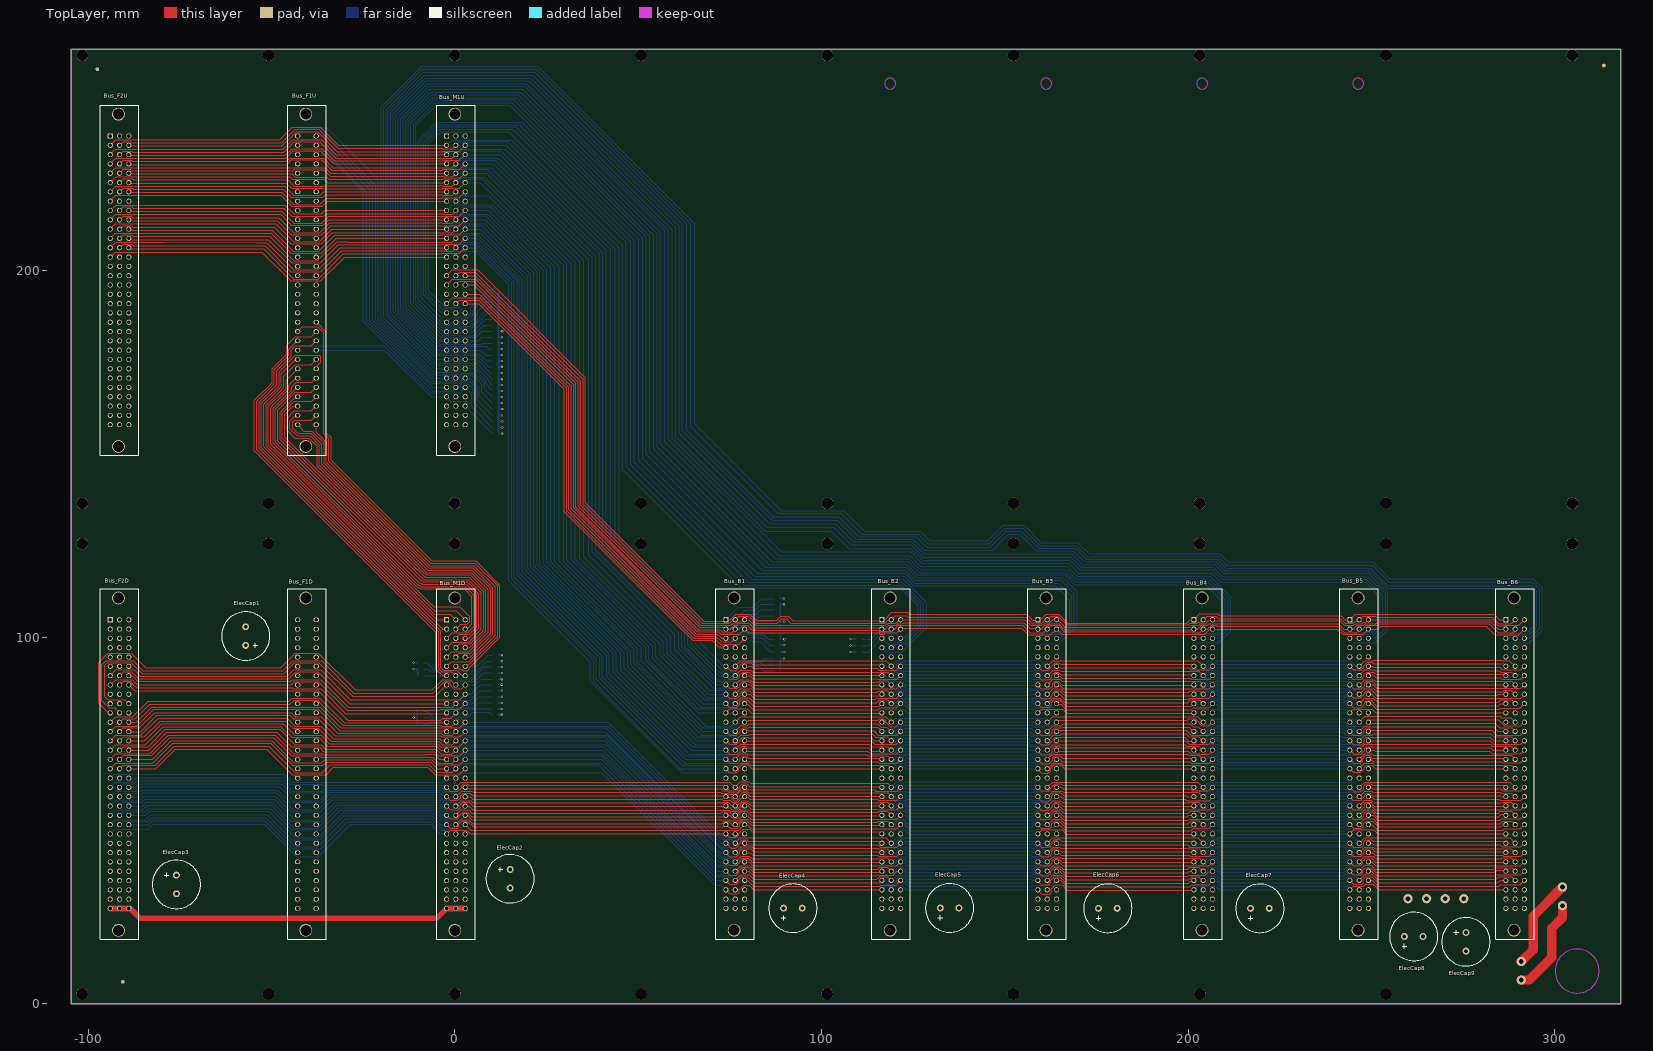
[diagram p0: TopLayer view]
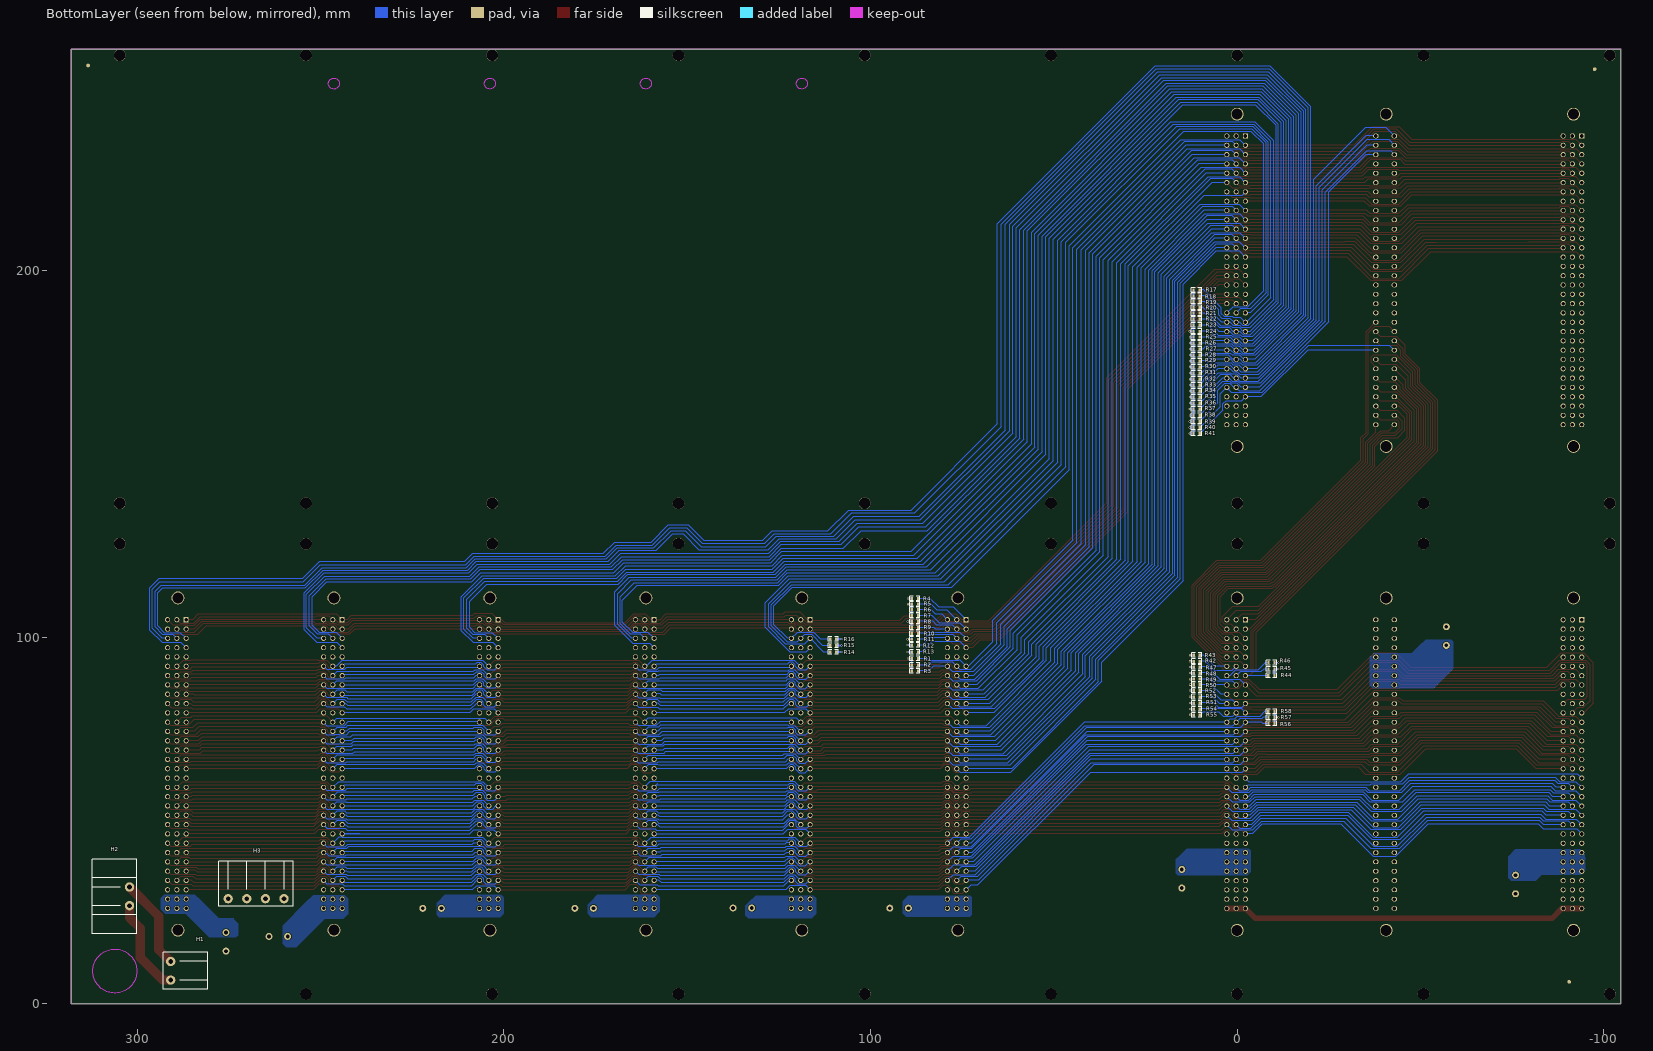
[diagram p1: BottomLayer view, seen from below]
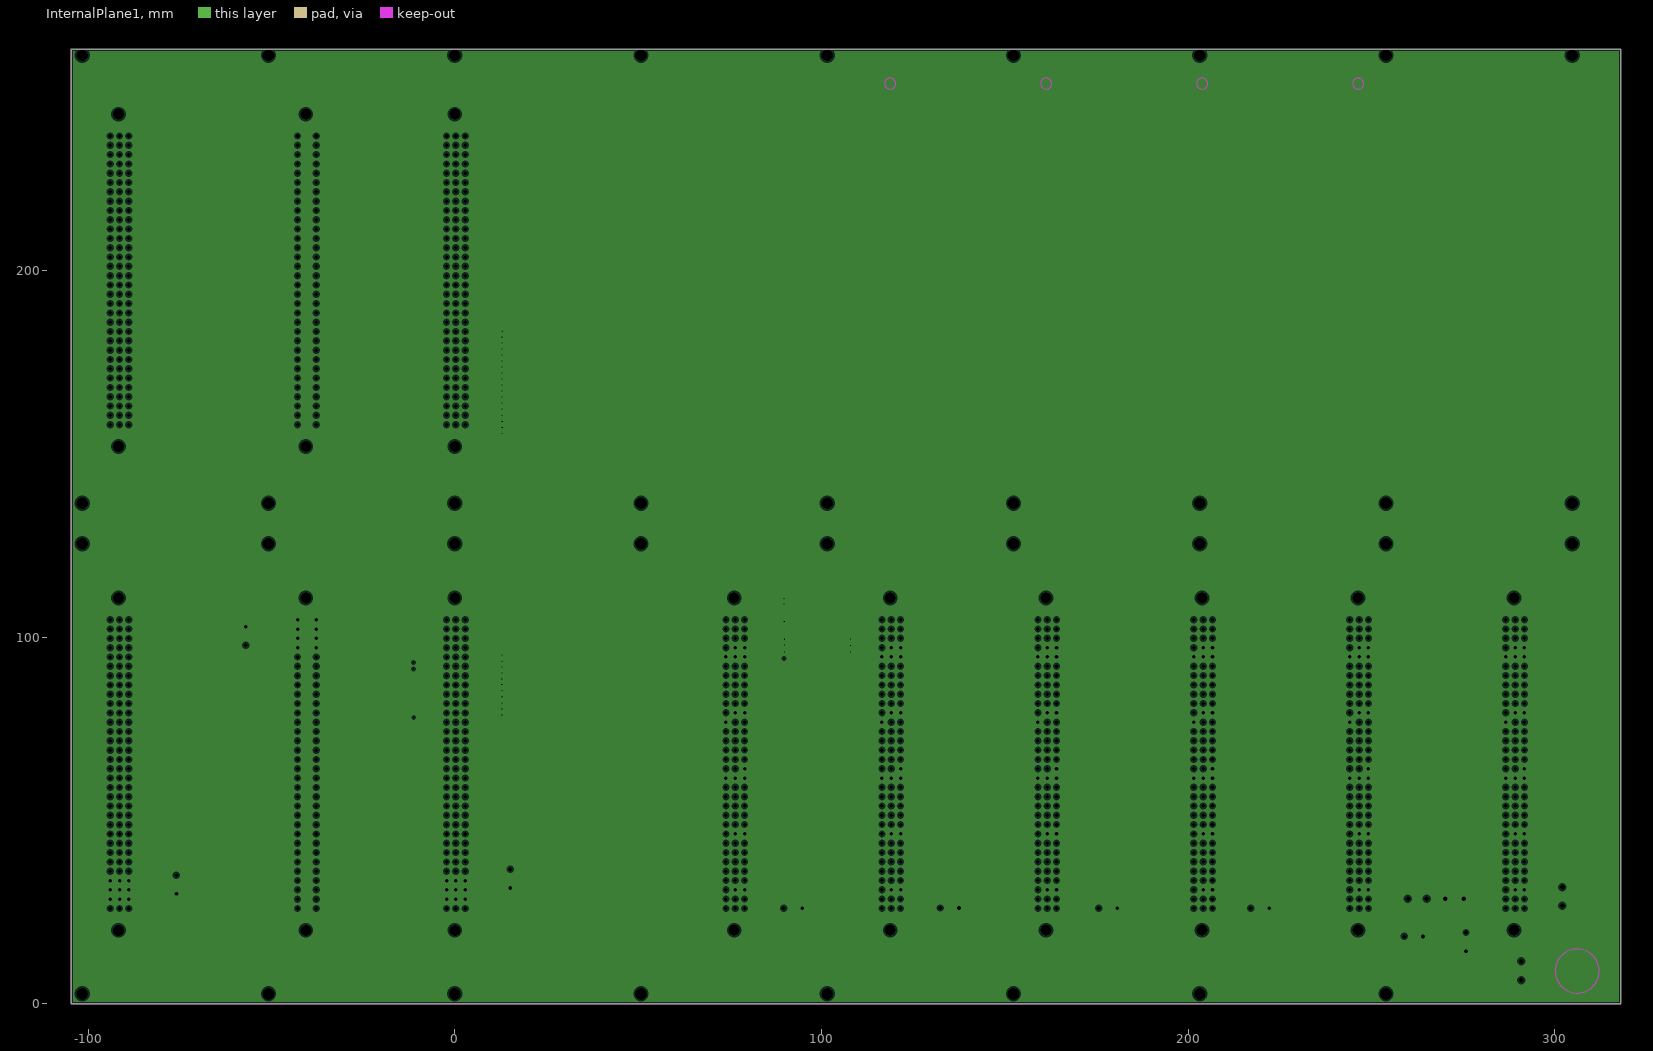
[diagram p2: InternalPlane1, clearances drawn from the general rule]
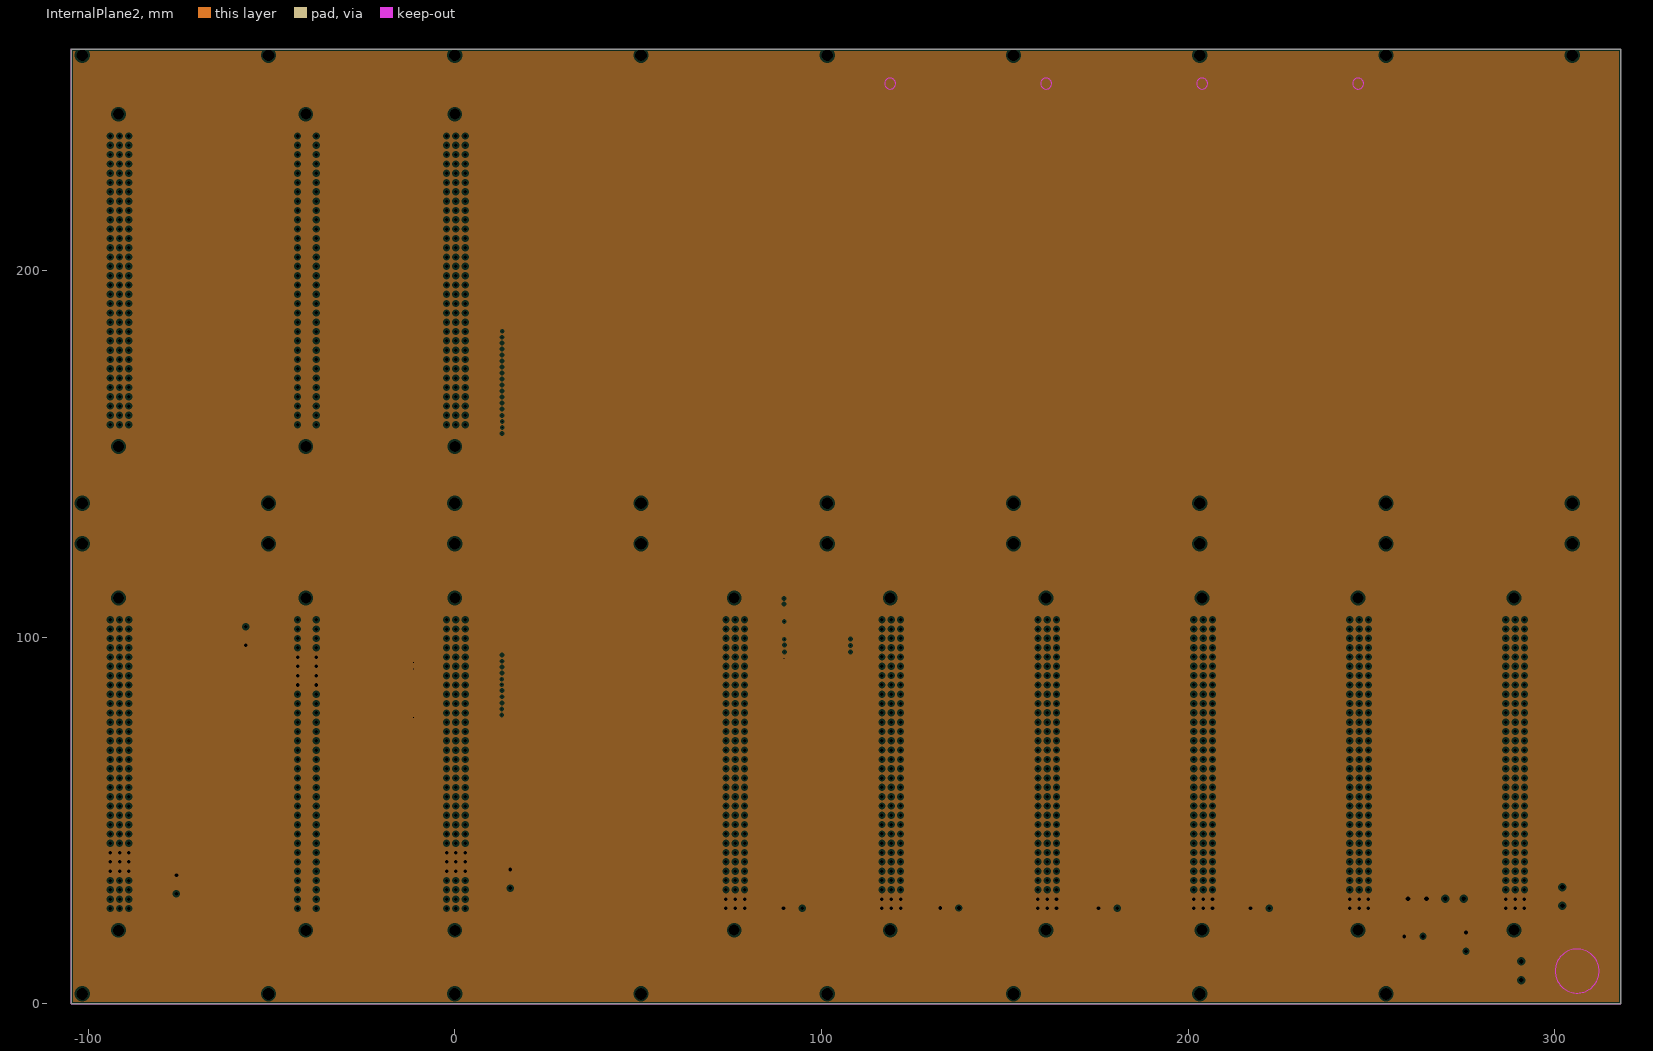
[diagram p3: InternalPlane2, clearances drawn from the general rule]
# Altium PCB MISC67337.PcbDoc (part 1 of 7)
Units mm, origin at the board's own origin, x right, y up, seen from the top; angles counter-clockwise.
Board outline 422.71 x 260.35 mm, 4 copper layers (TopLayer, InternalPlane1, InternalPlane2, BottomLayer); 82 components, 143 nets, 1295 pads, 42 vias.

## Layer stack, top to bottom (the 12.6 mil dielectric is the usual default, probably not edited)
TopLayer: signal copper 0.0356
Dielectric: core 0.32, FR-4, Dk 4.8
InternalPlane1: plane copper 0.0356, net GND
Dielectric: prepreg 0.32, FR-4, Dk 4.8
InternalPlane2: plane copper 0.0356, net +5V
Dielectric: core 0.32, FR-4, Dk 4.8
BottomLayer: signal copper 0.0356

## Board outline
-104.641,0 -104.641,260.35 318.066,260.35 318.066,0

## Design rules (kind name [scope] priority, off if disabled: settings)
Clearance [All] p1: gap=0.152
ComponentClearance [All] p1 off: gap=0.254 collisioncheckmode=3 verticalgap=0.254 showdistances=FALSE
FabricationTestPointUsage TestPointUsage [All] p1: valid=0 allowmultiple=FALSE
FabricationTestpoint Testpoint [All] p1: side=3 testpointundercomponent=TRUE minsize=1.016 maxsize=2.54 preferedsize=1.524 minholesize=0.508 maxholesize=1.016 preferedholesize=0.813 testpointgrid=0.025 allowsidetop=TRUE allowsidebottom=TRUE usegrid=TRUE gridtolerance=0
PlaneClearance [All] p1: clearance=0.508
PlaneConnect [All] p1: planeconnectstyle=Direct reliefexpansion=0.508 reliefentries=4 reliefconductorwidth=0.254 reliefairgap=0.254
PolygonConnect [All] p1: connectstyle=Relief reliefconductorwidth=0.254 reliefentries=4 polygonreliefangle="90 Angle"
RoutingVias [All] p1: holewidth=0.508 width=1.016 viastyle="Through Hole" minholewidth=0.305 minwidth=0.61 maxholewidth=0.711 maxwidth=1.27
SilkscreenOverComponentPads [All] p1: minsilkscreentomaskgap=0.254
SolderMaskExpansion [All] p1: expansion=0.102
Width [All] p1: maxlimit=25.4 minlimit=0.254 preferedwidth=0.254
22 further rules are at their usual default settings.

## Components (designator, comment, footprint, x,y, rotation, side; value= is the part's Value field where it differs from the comment)
Bus_B1 "OUPIIN Header32*3" OUPIINBUS32*3_ZHILI 76.195,110.663 r0 top locked
Bus_B2 "OUPIIN Header32*3" OUPIINBUS32*3_ZHILI 118.745,110.663 r0 top locked
Bus_B3 "OUPIIN Header32*3" OUPIINBUS32*3_ZHILI 161.29,110.663 r0 top locked
Bus_B4 "OUPIIN Header32*3" OUPIINBUS32*3_ZHILI 203.835,110.663 r0 top locked
Bus_B5 "OUPIIN Header32*3" OUPIINBUS32*3_ZHILI 246.38,110.663 r0 top locked
Bus_B6 "OUPIIN Header32*3" OUPIINBUS32*3_ZHILI 288.925,110.663 r0 top locked
Bus_F1D "CON64" OUPIINBUS32*2_ZHILI -40.64,110.644 r0 top locked
Bus_F1U "CON64" OUPIINBUS32*2_ZHILI -40.64,242.603 r0 top locked
Bus_F2D "OUPIIN Header32*3" OUPIINBUS32*3_ZHILI -91.73,110.644 r0 top locked
Bus_F2U "OUPIIN Header32*3" OUPIINBUS32*3_ZHILI -91.73,242.603 r0 top locked
Bus_M1D "OUPIIN Header32*3" OUPIINBUS32*3_ZHILI 0,110.644 r0 top locked
Bus_M1U "OUPIIN Header32*3" OUPIINBUS32*3_ZHILI 0,242.603 r0 top locked
ElecCap1 "1000uF/35V" 1000UF/35V -57.023,97.714 r270 top
ElecCap2 "1000uF/35V" 1000UF/35V 15.113,36.601 r90 top
ElecCap3 "1000uF/35V" 1000UF/35V -75.921,35.052 r90 top
ElecCap4 "1000uF/35V" 1000UF/35V 89.687,26.035 r180 top
ElecCap5 "1000uF/35V" 1000UF/35V 132.436,26.086 r180 top
ElecCap6 "1000uF/35V" 1000UF/35V 175.59,25.984 r180 top
ElecCap7 "1000uF/35V" 1000UF/35V 217.068,25.984 r180 top
ElecCap8 "1000uF/35V" 1000UF/35V 259.012,18.321 r180 top
ElecCap9 "1000uF/35V" 1000UF/35V 275.819,19.406 r90 top
H1 "Header2" EDGCon_2p_5.08mm 290.906,6.426 r90 bottom locked
H2 "Header2" EDGCON_2p_5.08mm_ear 302.133,26.721 r270 bottom locked
H3 "Header4" EDGCON_4p_5.08mm 265.074,28.626 r0 bottom
R1 "10k" 0603 88.773,94.132 r180 bottom
R2 "10k" 0603 87.097,92.38 r0 bottom
R3 "10k" 0603 88.773,90.754 r180 bottom
R4 "10k" 0603 88.773,110.49 r180 bottom
R5 "10k" 0603 87.097,108.991 r0 bottom
R6 "10k" 0603 88.773,107.442 r180 bottom
R7 "10k" 0603 88.773,105.842 r180 bottom
R8 "10k" 0603 87.097,104.242 r0 bottom
R9 "10k" 0603 88.773,102.565 r180 bottom
R10 "10k" 0603 88.773,100.965 r180 bottom
R11 "10k" 0603 88.773,99.39 r180 bottom
R12 "10k" 0603 87.097,97.79 r0 bottom
R13 "10k" 0603 88.773,95.936 r180 bottom
R14 "10k" 0603 109.372,95.885 r0 bottom
R15 "10k" 0603 111.049,97.663 r180 bottom
R16 "10k" 0603 109.372,99.441 r0 bottom
R17 "10k" 0603 11.938,194.666 r180 bottom
R18 "10k" 0603 10.262,193.065 r0 bottom
R19 "10k" 0603 11.938,191.491 r180 bottom
R20 "10k" 0603 11.938,189.916 r180 bottom
R21 "10k" 0603 10.262,188.316 r0 bottom
R22 "10k" 0603 11.938,186.69 r180 bottom
R23 "10k" 0603 11.938,185.064 r180 bottom
R24 "10k" 0603 10.262,183.388 r0 bottom
R25 "10k" 0603 11.938,181.762 r180 bottom
R26 "10k" 0603 11.938,180.162 r180 bottom
R27 "10k" 0603 10.262,178.537 r0 bottom
R28 "10k" 0603 11.938,176.886 r180 bottom
R29 "10k" 0603 11.938,175.311 r180 bottom
R30 "10k" 0603 10.262,173.685 r0 bottom
R31 "10k" 0603 11.938,171.983 r180 bottom
R32 "10k" 0603 11.938,170.332 r180 bottom
R33 "10k" 0603 10.262,168.732 r0 bottom
R34 "10k" 0603 11.938,167.107 r180 bottom
R35 "10k" 0603 11.938,165.481 r180 bottom
R36 "10k" 0603 10.262,163.805 r0 bottom
R37 "10k" 0603 11.938,162.154 r180 bottom
R38 "10k" 0603 11.938,160.452 r180 bottom
R39 "10k" 0603 10.262,158.775 r0 bottom
R40 "10k" 0603 11.938,157.124 r180 bottom
R41 "10k" 0603 11.938,155.473 r180 bottom
R42 "10k" 0603 10.185,93.37 r0 bottom
R43 "10k" 0603 11.862,95.047 r180 bottom
R44 "10k" 0603 -10.16,89.459 r0 bottom
R45 "10k" 0603 -8.509,91.237 r180 bottom
R46 "10k" 0603 -10.185,92.989 r0 bottom
R47 "10k" 0603 11.862,91.821 r180 bottom
R48 "10k" 0603 10.185,90.195 r0 bottom
R49 "10k" 0603 11.862,88.494 r180 bottom
R50 "10k" 0603 11.862,86.995 r180 bottom
R51 "10k" 0603 11.862,82.042 r180 bottom
R52 "10k" 0603 10.185,85.395 r0 bottom
R53 "10k" 0603 11.862,83.693 r180 bottom
R54 "10k" 0603 11.862,80.391 r180 bottom
R55 "10k" 0603 10.185,78.765 r0 bottom
R56 "10k" 0603 -10.185,76.378 r0 bottom
R57 "10k" 0603 -8.509,78.054 r180 bottom
R58 "10k" 0603 -10.16,79.705 r0 bottom

## Footprints (in the part's own frame and the unit in brackets; to place one, negate y for a bottom-side part, rotate by r counter-clockwise, add the part's x,y. Pads: shape width x height; smd on the part's side, far side on the other; paste and mask are expansions set on the pad)
0603 [mil]
  rect 25x32 smd: 1(0,0) 2(66,0)
  silkscreen extent -22,-25 88,25
1000UF/35V [mm]
  round 1.9 hole 1.016: 1(0,0) 2(-5.08,0)
  silkscreen extent -9.14,-6.6 4.06,6.6
EDGCon_2p_5.08mm [mil]
  round 100 hole 51: 1(0,0) 2(200,0)
  silkscreen extent -100,-400 300,80
EDGCON_2p_5.08mm_ear [mil]
  round 100 hole 51: 1(-200,0) 2(0,0)
  silkscreen extent -500,-400 300,80
EDGCON_4p_5.08mm [mil]
  round 100 hole 51: 1(-200,0) 2(0,0) 3(200,0) 4(400,0)
  silkscreen extent -300,-400 500,80
OUPIINBUS32*2_ZHILI [mm]
  round 3.5 hole 3: 0(0,-90.64) 0(0,0)
  oval 1.524x1.27 hole 0.965: A1(-2.24,-5.95) A2(-2.24,-8.49) A3(-2.24,-11.03) A4(-2.24,-13.57) A5(-2.24,-16.11) A6(-2.24,-18.65) A7(-2.24,-21.19) A8(-2.24,-23.73) A9(-2.24,-26.27) A10(-2.24,-28.81) A11(-2.24,-31.35) A12(-2.24,-33.89) A13(-2.24,-36.43) A14(-2.24,-38.97) A15(-2.24,-41.51) A16(-2.24,-44.05) A17(-2.24,-46.59) A18(-2.24,-49.13) A19(-2.24,-51.67) A20(-2.24,-54.21) A21(-2.24,-56.75) A22(-2.24,-59.29) A23(-2.24,-61.83) A24(-2.24,-64.37) A25(-2.24,-66.91) A26(-2.24,-69.45) A27(-2.24,-71.99) A28(-2.24,-74.53) A29(-2.24,-77.07) A30(-2.24,-79.61) A31(-2.24,-82.15) A32(-2.24,-84.69) C1(2.84,-5.95) C2(2.84,-8.49) C3(2.84,-11.03) C4(2.84,-13.57) C5(2.84,-16.11) C6(2.84,-18.65) C7(2.84,-21.19) C8(2.84,-23.73) C9(2.84,-26.27) C10(2.84,-28.81) C11(2.84,-31.35) C12(2.84,-33.89) C13(2.84,-36.43) C14(2.84,-38.97) C15(2.84,-41.51) C16(2.84,-44.05) C17(2.84,-46.59) C18(2.84,-49.13) C19(2.84,-51.67) C20(2.84,-54.21) C21(2.84,-56.75) C22(2.84,-59.29) C23(2.84,-61.83) C24(2.84,-64.37) C25(2.84,-66.91) C26(2.84,-69.45) C27(2.84,-71.99) C28(2.84,-74.53) C29(2.84,-77.07) C30(2.84,-79.61) C31(2.84,-82.15) C32(2.84,-84.69)
  silkscreen extent -4.95,-93.09 5.55,2.45
OUPIINBUS32*3_ZHILI [mil]
  round 137.79 hole 118.11: 0(0,-3568.5) 0(0,0)
  rect 55x55 hole 38: A1(-88.19,-234.25)
  round 55 hole 38: A2(-88.19,-334.25) A3(-88.19,-434.25) A4(-88.19,-534.25) A5(-88.19,-634.25) A6(-88.19,-734.25) A7(-88.19,-834.25) A8(-88.19,-934.25) A9(-88.19,-1034.25) A10(-88.19,-1134.25) A11(-88.19,-1234.25) A12(-88.19,-1334.25) A13(-88.19,-1434.25) A14(-88.19,-1534.25) A15(-88.19,-1634.25) A16(-88.19,-1734.25) A17(-88.19,-1834.25) A18(-88.19,-1934.25) A19(-88.19,-2034.25) A20(-88.19,-2134.25) A21(-88.19,-2234.25) A22(-88.19,-2334.25) A23(-88.19,-2434.25) A24(-88.19,-2534.25) A25(-88.19,-2634.25) A26(-88.19,-2734.25) A27(-88.19,-2834.25) A28(-88.19,-2934.25) A29(-88.19,-3034.25) A30(-88.19,-3134.25) A31(-88.19,-3234.25) A32(-88.19,-3334.25) B1(11.81,-234.25) B2(11.81,-334.25) B3(11.81,-434.25) B4(11.81,-534.25) B5(11.81,-634.25) B6(11.81,-734.25) B7(11.81,-834.25) B8(11.81,-934.25) B9(11.81,-1034.25) B10(11.81,-1134.25) B11(11.81,-1234.25) B12(11.81,-1334.25) B13(11.81,-1434.25) B14(11.81,-1534.25) B15(11.81,-1634.25) B16(11.81,-1734.25) B17(11.81,-1834.25) B18(11.81,-1934.25) B19(11.81,-2034.25) B20(11.81,-2134.25) B21(11.81,-2234.25) B22(11.81,-2334.25) B23(11.81,-2434.25) B24(11.81,-2534.25) B25(11.81,-2634.25) B26(11.81,-2734.25) B27(11.81,-2834.25) B28(11.81,-2934.25) B29(11.81,-3034.25) B30(11.81,-3134.25) B31(11.81,-3234.25) B32(11.81,-3334.25) C1(111.81,-234.25) C2(111.81,-334.25) C3(111.81,-434.25) C4(111.81,-534.25) C5(111.81,-634.25) C6(111.81,-734.25) C7(111.81,-834.25) C8(111.81,-934.25) C9(111.81,-1034.25) C10(111.81,-1134.25) C11(111.81,-1234.25) C12(111.81,-1334.25) C13(111.81,-1434.25) C14(111.81,-1534.25) C15(111.81,-1634.25) C16(111.81,-1734.25) C17(111.81,-1834.25) C18(111.81,-1934.25) C19(111.81,-2034.25) C20(111.81,-2134.25) C21(111.81,-2234.25) C22(111.81,-2334.25) C23(111.81,-2434.25) C24(111.81,-2534.25) C25(111.81,-2634.25) C26(111.81,-2734.25) C27(111.81,-2834.25) C28(111.81,-2934.25) C29(111.81,-3034.25) C30(111.81,-3134.25) C31(111.81,-3234.25) C32(111.81,-3334.25)
  silkscreen extent -195,-3665 219,96

## Part data
ElecCap1 ElecCap2 ElecCap3 ElecCap4 ElecCap5 ElecCap6 ElecCap7 ElecCap8 ElecCap9: library part ELECTROCap, "Electrolytic Capacitor(Pin1 Positive)"
R1 R2 R3 R4 R5 R6 R7 R8 R9 R10 R11 R12 R13 R14 R15 R16 R17 R18 R19 R20 R21 R22 R23 R24 R25 R26 R27 R28 R29 R30 R31 R32 R33 R34 R35 R36 R37 R38 R39 R40 R41 R42 R43 R44 R45 R46 R47 R48 R49 R50 R51 R52 R53 R54 R55 R56 R57 R58: library part RES2

## Free pads (board coordinates)
  round 1 smd far side mask+1: 0(-97.485,254.889) 0(-90.526,5.944) 0(313.436,255.88)
  round 1 smd mask+1: 0(-97.485,254.889) 0(-90.526,5.944) 0(313.436,255.88)
  round 3.2 hole 3.2: 0(0,2.642) 0(0,125.471) 0(0,136.469) 0(0,258.642) 1(-50.8,2.642) 1(-50.8,125.471) 1(-50.8,136.469) 1(-50.8,258.642) 1(50.8,2.642) 1(50.8,125.471) 1(50.8,136.469) 1(50.8,258.642) 2(-101.6,2.642) 2(-101.6,125.471) 2(-101.6,136.469) 2(-101.6,258.642) 2(101.6,2.642) 2(101.6,125.471) 2(101.6,136.469) 2(101.6,258.642) 3(152.4,2.642) 3(152.4,125.471) 3(152.4,136.469) 3(152.4,258.642) 4(203.2,2.642) 4(203.2,125.471) 4(203.2,136.469) 4(203.2,258.642) 5(254,2.642) 5(254,125.471) 5(254,136.469) 5(254,258.642) 6(304.8,125.471) 6(304.8,136.469) 6(304.8,258.642)

## Via types
v1: diameter 0.61, hole 0.305, TopLayer to BottomLayer, 42 vias

## Nets (pads, with @x,y where several pads share a name; then routed paths per layer and width w, separated by ;. In a path a pad name is that pad's centre, name@x,y a point inside that pad or via, vN(x,y) a via of type N, cw(c..) or ccw(c..) an arc to the next point about the centre after c; other vN are vias at no path point)
+5V: Bus_B1.A31 Bus_B1.A32 Bus_B1.B31 Bus_B1.B32 Bus_B1.C31 Bus_B1.C32 Bus_B2.A31 Bus_B2.A32 Bus_B2.B31 Bus_B2.B32 Bus_B2.C31 Bus_B2.C32 Bus_B3.A31 Bus_B3.A32 Bus_B3.B31 Bus_B3.B32 Bus_B3.C31 Bus_B3.C32 Bus_B4.A31 Bus_B4.A32 Bus_B4.B31 Bus_B4.B32 Bus_B4.C31 Bus_B4.C32 Bus_B5.A31 Bus_B5.A32 Bus_B5.B31 Bus_B5.B32 Bus_B5.C31 Bus_B5.C32 Bus_B6.A31 Bus_B6.A32 Bus_B6.B31 Bus_B6.B32 Bus_B6.C31 Bus_B6.C32 Bus_F1D.A5 Bus_F1D.A6 Bus_F1D.A7 Bus_F1D.A8 Bus_F1D.C5 Bus_F1D.C6 Bus_F1D.C7 Bus_F1D.C8 Bus_F2D.A26 Bus_F2D.A27 Bus_F2D.A28 Bus_F2D.B26 Bus_F2D.B27 Bus_F2D.B28 Bus_F2D.C26 Bus_F2D.C27 Bus_F2D.C28 Bus_M1D.A26 Bus_M1D.A27 Bus_M1D.A28 Bus_M1D.B26 Bus_M1D.B27 Bus_M1D.B28 Bus_M1D.C26 Bus_M1D.C27 Bus_M1D.C28 ElecCap1.1 ElecCap2.1 ElecCap3.1 ElecCap4.1 ElecCap5.1 ElecCap6.1 ElecCap7.1 ElecCap8.1 ElecCap9.1 H3.1 H3.2 R1.1 R2.2 R3.1 R44.1 R45.2 R46.1 R56.1 R57.2 R58.1 | length 12.8
  BottomLayer w0.381: v1(-11.252,91.262) -11.227,91.237 R45.2@-10.185,91.237 -10.16,91.211 R44.1@-10.16,89.459 ; v1(-11.227,93.015) -11.201,92.989 R46.1@-10.185,92.989 ; v1(-11.201,78.054) R57.2@-10.185,78.054 ; R56.1@-10.185,76.378 R57.2@-10.185,78.054 ; R58.1@-10.16,79.705 -10.185,79.68 R57.2@-10.185,78.054 ; R3.1@88.773,90.754 R2.2@88.773,92.38 R1.1@88.773,94.132 89.687,94.132 89.789,94.234 89.814,94.209 v1(89.814,94.132)
AC1: H1.1 H2.2 | length 26.2
  TopLayer w2.54: H1.1@290.906,6.426 293.065,6.426 299.212,12.573 299.212,20.574 302.133,23.495 H2.2@302.133,26.721
AC2: H1.2 H2.1 | length 24.9
  TopLayer w2.54: H1.2@290.906,11.506 294.132,14.732 294.132,23.8 H2.1@302.133,31.801
AD_BUSY1: Bus_F1U.A24 Bus_M1U.C28 R40.2 | length 66.1
  BottomLayer w0.254: Bus_F1U.A24@-42.88,178.233 -41.662,179.451 -19.406,179.451 -6.644,166.689 1.456,166.689 Bus_M1U.C28@2.84,168.073 4.572,166.341 4.572,162.814 R40.2@10.262,157.124
AD_BUSY2: Bus_F1U.C24 Bus_M1U.A29 R41.2 | length 58.5
  BottomLayer w0.254: Bus_F1U.C24@-37.8,178.233 -19.179,178.233 -6.479,165.533 Bus_M1U.A29@-2.24,165.533 -1.045,164.338 3.175,164.338 3.937,163.576 3.937,161.798 R41.2@10.262,155.473
AD_CON: Bus_F1U.C21 Bus_M1D.B6 R42.1 | length 141.6
  TopLayer w0.254: Bus_F1U.C21@-37.8,185.853 -37.699,185.853 -35.128,183.283 -35.128,155.686 -33.731,154.289 -33.731,148.218 -6.265,120.752 5.745,120.752 12.319,114.178 12.319,99.987 4.046,91.715 4.046,91.494 3.34,90.788 2.34,90.788 1.967,91.161 1.177,91.161 0.344,91.994 Bus_M1D.B6@0.3,91.994
  BottomLayer w0.254: Bus_M1D.B6@0.3,91.994 1.489,90.805 6.096,90.805 8.661,93.37 R42.1@10.185,93.37
AD_CS: Bus_F1U.C23 Bus_M1D.C7 R46.2 | length 139
  TopLayer w0.254: Bus_F1U.C23@-37.8,180.773 -39.197,179.376 -43.48,179.376 -44.577,178.28 -44.577,176.638 -48.565,172.65 -48.565,168.804 -53.365,164.004 -53.365,151.3 -3.81,101.745 -3.81,91.669 -3.073,90.932 0.508,90.932 1.986,89.454 Bus_M1D.C7@2.84,89.454
  BottomLayer w0.254: R46.2@-8.509,92.989 -7.645,92.989 -5.588,90.932 0.508,90.932 1.986,89.454 Bus_M1D.C7@2.84,89.454
AD_D0: Bus_F1U.A25 Bus_M1D.A1 | length 97.5
  TopLayer w0.254: Bus_F1U.A25@-42.954,175.767 Bus_F1U.A25@-42.88,175.693 -43.382,175.693 -47.295,171.78 -47.295,168.278 -52.095,163.478 -52.095,151.826 -4.963,104.694 Bus_M1D.A1@-2.24,104.694
AD_D1: Bus_F1U.C25 Bus_M1D.B1 | length 103.2
  TopLayer w0.254: Bus_F1U.C25@-37.8,175.693 -39.197,174.296 -43.48,174.296 -46.66,171.117 -46.66,168.015 -51.46,163.215 -51.46,152.09 -51.283,151.912 -5.543,106.172 -1.178,106.172 Bus_M1D.B1@0.3,104.694
AD_D2: Bus_F1U.A26 Bus_M1D.C1 | length 97.5
  TopLayer w0.254: Bus_F1U.A26@-42.88,173.153 -46.025,170.009 -46.025,167.752 -50.825,162.952 -50.825,152.353 -48.754,150.281 -5.661,107.188 0.346,107.188 Bus_M1D.C1@2.84,104.694
AD_D3: Bus_F1U.C26 Bus_M1D.A2 | length 111
  TopLayer w0.254: Bus_F1U.C26@-37.8,173.153 -37.8,173.604 -36.525,174.879 -36.525,176.403 -36.959,176.836 -43.48,176.836 -47.93,172.387 -47.93,168.541 -52.73,163.741 -52.73,151.563 -50.053,148.886 -3.321,102.154 Bus_M1D.A2@-2.24,102.154
AD_D4: Bus_F1U.A27 Bus_M1D.B2 | length 101
  TopLayer w0.254: Bus_F1U.A27@-42.88,170.613 -43.356,170.613 -45.237,168.732 -45.237,167.642 -50.19,162.689 -50.19,152.616 -5.779,108.204 1.422,108.204 4.046,105.58 4.046,104.194 3.34,103.488 2.34,103.488 2.323,103.505 1.651,103.505 Bus_M1D.B2@0.3,102.154
AD_D5: Bus_F1U.C27 Bus_M1D.C2 | length 106.6
  TopLayer w0.254: Bus_F1U.C27@-37.8,170.613 -38.943,169.47 -43.226,169.47 -44.501,168.196 -44.501,167.48 -49.555,162.426 -49.555,152.879 -10.215,113.538 -9.827,113.538 -9.421,113.132 2.589,113.132 4.681,111.039 4.681,103.497 3.514,102.329 3.514,102.32 3.348,102.154 Bus_M1D.C2@2.84,102.154
AD_D6: Bus_F1U.A28 Bus_M1D.A3 | length 106.4
  TopLayer w0.254: Bus_F1U.A28@-42.88,168.073 -43.01,168.073 -48.92,162.163 -48.92,153.142 -9.952,114.173 -9.564,114.173 -9.158,113.767 2.852,113.767 5.316,111.302 5.316,102.924 3.51,101.117 -0.737,101.117 Bus_M1D.A3@-2.24,99.614
AD_D7: Bus_F1U.C28 Bus_M1D.B3 | length 109
  TopLayer w0.254: -47.529,152.648 -48.285,153.405 -48.285,161.9 -43.485,166.7 -39.173,166.7 Bus_F1U.C28@-37.8,168.073 ; -47.511,152.667 -9.652,114.808 -9.301,114.808 -8.895,114.402 3.115,114.402 5.951,111.565 5.951,102.661 4.001,100.711 ; Bus_M1D.B3@0.3,99.614 1.397,100.711 4.001,100.711 ; 3.931,100.641 4.001,100.711
AD_D8: Bus_F1U.A29 Bus_M1D.C3 | length 100
  TopLayer w0.254: Bus_F1U.A29@-42.88,165.533 -43.4,165.533 -47.65,161.283 -47.65,153.822 -9.271,115.443 -9.038,115.443 -8.632,115.037 3.378,115.037 6.604,111.811 6.604,102.387 3.831,99.614 Bus_M1D.C3@2.84,99.614
AD_D9: Bus_F1U.C29 Bus_M1D.A4 | length 111
  TopLayer w0.254: -44.407,163.628 -47.015,161.02 -47.015,154.194 -8.899,116.078 ; -44.398,163.628 -43.764,164.262 -39.072,164.262 Bus_F1U.C29@-37.8,165.533 ; -8.775,116.078 -8.369,115.672 3.641,115.672 7.239,112.074 7.239,102.124 3.751,98.636 -0.678,98.636 Bus_M1D.A4@-2.24,97.074
AD_D10: Bus_F1U.A30 Bus_M1D.B4 | length 102.5
  TopLayer w0.254: Bus_F1U.A30@-42.88,162.993 -44.144,162.993 -46.38,160.757 -46.38,154.457 -41.987,150.064 -41.934,150.064 -41.575,149.705 -41.575,149.703 -10.363,118.491 -10.296,118.491 -8.518,116.713 -8.512,116.713 -8.106,116.307 3.904,116.307 7.874,112.337 7.874,101.861 4.216,98.204 4.216,98.171 1.397,98.171 Bus_M1D.B4@0.3,97.074
AD_D11: Bus_F1U.C30 Bus_M1D.C4 | length 106.8
  TopLayer w0.254: Bus_F1U.C30@-37.8,162.993 -39.097,161.696 -43.764,161.696 -45.745,159.715 -45.745,156.337 -43.63,154.221 -39.705,154.221 -37.541,152.058 -37.541,146.64 -10.535,119.634 -10.535,119.628 -8.255,117.348 -8.249,117.348 -7.843,116.942 4.167,116.942 8.509,112.6 8.509,101.598 4.851,97.941 4.851,97.908 4.017,97.074 Bus_M1D.C4@2.84,97.074
AD_D12: Bus_F1U.A31 Bus_M1D.A5 | length 106
  TopLayer w0.254: Bus_F1U.A31@-42.88,160.453 -43.382,160.453 -44.983,158.852 -44.983,156.861 -42.986,154.864 -39.449,154.864 -36.906,152.321 -36.906,146.903 -7.58,117.577 4.43,117.577 9.144,112.863 9.144,101.335 5.486,97.678 5.486,97.645 3.988,96.147 3.734,96.147 ; Bus_M1D.A5@-2.24,94.534 -0.762,96.012 3.734,96.012
AD_D13: Bus_F1U.C31 Bus_M1D.B5 | length 108.4
  TopLayer w0.254: Bus_F1U.C31@-37.8,160.453 -39.197,159.056 -43.712,159.056 -44.196,158.572 -44.196,156.972 -42.774,155.55 -39.237,155.55 -36.271,152.584 -36.271,147.166 -7.317,118.212 4.693,118.212 9.779,113.126 9.779,101.072 6.195,97.488 6.195,97.455 4.23,95.491 4.111,95.491 ; Bus_M1D.B5@0.3,94.534 1.278,95.512 4.111,95.512
AD_D14: Bus_F1U.A32 Bus_M1D.C5 | length 97.7
  TopLayer w0.254: Bus_F1U.A32@-42.88,157.913 -41.151,156.185 -38.974,156.185 -35.636,152.847 -35.636,147.429 -7.054,118.847 4.956,118.847 10.414,113.389 10.414,100.809 6.83,97.225 6.83,97.192 4.172,94.534 Bus_M1D.C5@2.84,94.534
AD_D15: Bus_F1U.C32 Bus_M1D.A6 | length 101.5
  TopLayer w0.254: Bus_F1U.C32@-37.8,157.913 -37.8,155.909 -35.001,153.11 -35.001,147.692 -6.791,119.482 5.219,119.482 11.049,113.652 11.049,100.513 3.754,93.218 -1.016,93.218 Bus_M1D.A6@-2.24,91.994
AD_RD1: Bus_F1U.C22 Bus_M1D.A7 R44.2 | length 131.9
  TopLayer w0.254: Bus_F1U.C22@-37.8,183.313 -39.197,181.916 -43.48,181.916 -45.847,179.55 -45.847,177.164 -49.835,173.176 -49.835,169.33 -54.635,164.53 -54.635,150.774 -5.131,101.27 -5.131,91.262 -3.323,89.454 Bus_M1D.A7@-2.24,89.454
  BottomLayer w0.254: R44.2@-8.484,89.459 -8.479,89.454 Bus_M1D.A7@-2.24,89.454
AD_RD2: Bus_F1U.A23 Bus_M1D.B7 R45.1 | length 129.7
  TopLayer w0.254: Bus_F1U.A23@-42.88,180.773 -42.981,180.773 -45.212,178.543 -45.212,176.901 -49.2,172.913 -49.2,169.067 -54,164.267 -54,151.037 -4.42,101.457 -4.42,91.389 -3.556,90.526 -0.772,90.526 Bus_M1D.B7@0.3,89.454
  BottomLayer w0.254: R45.1@-8.509,91.237 -7.188,91.237 -6.477,90.526 -0.772,90.526 Bus_M1D.B7@0.3,89.454
AD_RST: Bus_F1U.A22 Bus_M1D.C6 R43.2 | length 138.6
  TopLayer w0.254: Bus_F1U.A22@-42.88,183.313 -41.612,184.582 -37.325,184.582 -35.763,183.02 -35.763,155.423 -34.366,154.026 -34.366,147.955 -6.528,120.117 5.482,120.117 11.684,113.915 11.684,100.25 3.428,91.994 Bus_M1D.C6@2.84,91.994
  BottomLayer w0.254: Bus_M1D.C6@2.84,91.994 6.142,91.994 9.195,95.047 R43.2@10.185,95.047
B_DSP1_C\S\: Bus_B1.A25 Bus_B2.A25 Bus_B3.A25 Bus_B4.A25 Bus_B5.A25 Bus_B6.A25 Bus_F2D.A12 Bus_M1D.A12 R56.2 | length 428.5
  TopLayer w0.254: Bus_F2D.A12@-93.97,76.754 -92.492,78.232 -87.808,78.232 -83.617,82.423 -45.263,82.423 -44.374,83.312 -36.855,83.312 -30.124,76.581 -2.413,76.581 Bus_M1D.A12@-2.24,76.754 ; Bus_B1.A25@73.96,43.753 Bus_B1.A25@74.023,43.817 ; Bus_B1.A25@73.96,43.88 Bus_B1.A25@74.023,43.817 ; 114.136,44.268 113.538,44.268 ; Bus_B2.A25@116.505,43.753 115.99,44.268 113.538,44.268 ; Bus_B3.A25@159.05,43.626 Bus_B3.A25@159.113,43.69 ; Bus_B3.A25@159.05,43.753 Bus_B3.A25@159.113,43.69 ; 199.074,44.26 197.383,44.26 ; Bus_B4.A25@201.595,43.753 201.088,44.26 197.383,44.26 ; Bus_B5.A25@244.14,43.753 245.221,42.672 247.269,42.672 247.904,43.307 247.904,44.069 248.539,44.704 248.788,44.704 248.815,44.731 250.057,44.731 250.52,44.268 283.972,44.268 ; 285.707,44.268 283.972,44.268 ; Bus_B6.A25@286.685,43.753 286.17,44.268 283.972,44.268 ; Bus_B1.A25@74.023,43.817 75.422,42.418 76.581,42.418 78.057,43.894 78.057,44.28 78.508,44.731 79.649,44.731 80.112,44.268 113.538,44.268 ; Bus_B3.A25@159.113,43.69 160.131,42.672 162.052,42.672 163.152,43.772 163.152,44.158 163.825,44.831 164.936,44.831 165.506,44.26 197.383,44.26
  BottomLayer w0.254: R56.2@-8.509,76.378 -7.061,76.378 -6.685,76.754 Bus_M1D.A12@-2.24,76.754 -0.797,75.311 41.148,75.311 72.706,43.753 Bus_B1.A25@73.955,43.753 ; Bus_B2.A25@116.632,43.815 116.632,43.704 117.602,42.734 119.634,42.734 120.396,43.496 120.396,44.131 121.058,44.793 122.276,44.793 122.711,44.358 126.39,44.358 ; 124.422,44.358 126.39,44.358 ; 152.146,44.358 150.673,44.358 ; Bus_B3.A25@159.05,43.753 158.445,44.358 150.673,44.358 ; Bus_B4.A25@201.595,43.753 201.595,43.642 202.565,42.672 204.597,42.672 205.359,43.434 205.359,44.069 206.021,44.731 208.075,44.731 208.476,44.33 211.912,44.33 ; 209.385,44.33 211.912,44.33 ; 237.109,44.33 235.636,44.33 ; Bus_B5.A25@244.14,43.753 243.563,44.33 235.636,44.33 ; 126.39,44.358 150.673,44.358 ; 211.912,44.33 235.636,44.33
B_DSP1_X\R\D\: Bus_B1.B25 Bus_B2.B25 Bus_B3.B25 Bus_B4.B25 Bus_B5.B25 Bus_B6.B25 Bus_F2D.B12 Bus_M1D.B12 R57.1 | length 421.9
  TopLayer w0.254: Bus_F2D.B12@-91.43,76.754 -90.452,77.732 -87.089,77.732 -83.161,81.659 -44.985,81.659 -43.84,82.804 -37.35,82.804 -36.759,82.213 -36.759,82.098 -30.528,75.867 -3.683,75.867 -3.508,75.692 -0.762,75.692 Bus_M1D.B12@0.3,76.754 ; Bus_B1.B25@76.5,43.88 77.832,45.212 117.586,45.212 Bus_B2.B25@119.045,43.753 ; Bus_B3.B25@161.59,43.753 163.074,45.237 202.651,45.237 Bus_B4.B25@204.135,43.753 ; Bus_B5.B25@246.68,43.753 248.139,45.212 287.766,45.212 Bus_B6.B25@289.225,43.753
  BottomLayer w0.254: R57.1@-8.509,78.054 -7.061,78.054 -6.739,77.732 -0.678,77.732 Bus_M1D.B12@0.3,76.754 1.337,75.717 41.756,75.717 72.668,44.806 75.443,44.806 Bus_B1.B25@76.495,43.753 ; Bus_B2.B25@119.045,43.753 120.6,45.308 125.857,45.308 ; 123.698,45.308 125.857,45.308 ; 152.908,45.308 150.647,45.308 ; Bus_B3.B25@161.59,43.753 160.035,45.308 150.647,45.308 ; Bus_B3.B25@161.684,43.848 Bus_B3.B25@161.717,43.815 ; Bus_B4.B25@204.135,43.753 205.66,45.278 210.49,45.278 236.245,45.278 ; 237.871,45.278 236.245,45.278 ; Bus_B5.B25@246.68,43.753 245.118,45.315 244.069,45.315 244.032,45.278 236.245,45.278 ; 125.857,45.308 150.647,45.308